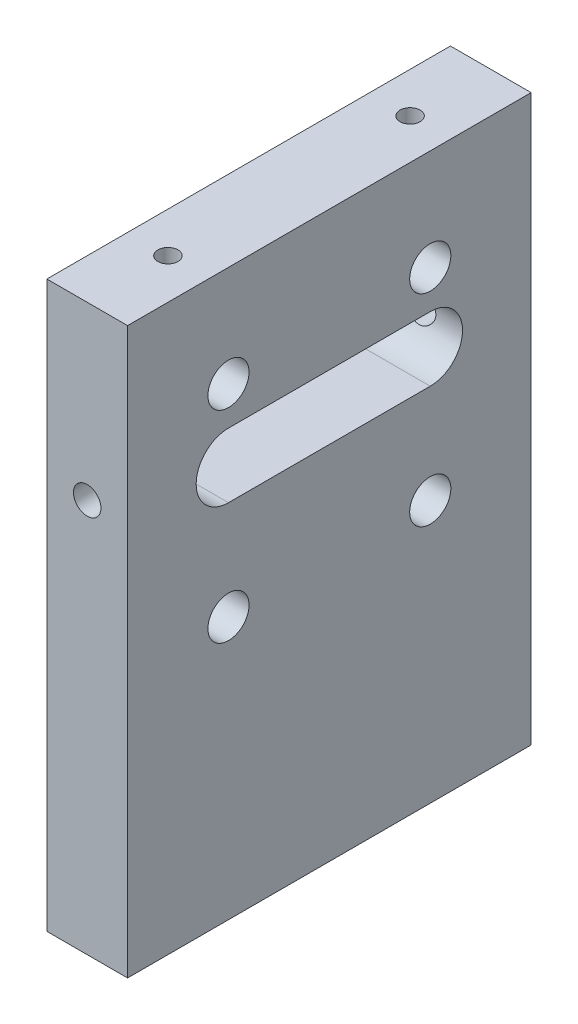
from build123d import *

# Parameters (mm, degrees)
SKETCH_1_W                    = 100
SKETCH_1_H                    = 140
EXTRUDE_1_DEPTH               = 20
HOLE_WIZARD_M6_1_D            = 5
HOLE_WIZARD_M6_1_DEPTH        = 15
HOLE_WIZARD_M6_1_TIP          = 1.502151548
CUT_EXTRUDE_1_DEPTH           = 89.317608663
HOLE_WIZARD_M8_1_D            = 6.8
HOLE_WIZARD_M12_1_D           = 10.2
HOLE_WIZARD_M12_1_CSINK_D     = 12.05
HOLE_WIZARD_M12_1_CSINK_ANGLE = 90
HOLE_WIZARD_M6_2_D            = 5
HOLE_WIZARD_M6_2_DEPTH        = 15
HOLE_WIZARD_M6_2_TIP          = 1.502151548


with BuildPart() as part:
    # 草图1 → 凸台-拉伸1 (new body)
    with BuildSketch(Plane(origin=(0, 0, 0), x_dir=(0, 0, -1), z_dir=(1, 0, 0))):
        Rectangle(SKETCH_1_W, SKETCH_1_H)
    extrude(amount=EXTRUDE_1_DEPTH)

    # M6 螺纹孔1
    with Locations(Plane(origin=(0, -70, 0), x_dir=(-1, 0, 0), z_dir=(0, -1, 0))):
        with Locations((-10, 30), (-10, -30)):
            Hole(HOLE_WIZARD_M6_1_D / 2, depth=HOLE_WIZARD_M6_1_DEPTH)
            with Locations((0, 0, -(HOLE_WIZARD_M6_1_DEPTH + HOLE_WIZARD_M6_1_TIP / 2))):  # 118° drill point
                Cone(0, HOLE_WIZARD_M6_1_D / 2, HOLE_WIZARD_M6_1_TIP, mode=Mode.SUBTRACT)

    # 草图4 → 切除-拉伸1 (cut, through all)
    with BuildSketch(Plane.ZY):
        with BuildLine():
            Line((-25, 35.5), (25, 35.5))
            ThreePointArc((25, 35.5), (33, 27.5), (25, 19.5))
            Line((25, 19.5), (-25, 19.5))
            ThreePointArc((-25, 19.5), (-33, 27.5), (-25, 35.5))
        make_face()
    extrude(amount=-CUT_EXTRUDE_1_DEPTH, mode=Mode.SUBTRACT)

    # M8 螺纹孔1 (through all)
    with Locations(Plane.XY.offset(50)):
        with Locations((10, 27.5)):
            Hole(HOLE_WIZARD_M8_1_D / 2)

    # M12 螺纹孔1 (through all)
    with Locations(Plane.ZY):
        with Locations((-25, 45), (25, 45), (-25, -5), (25, -5)):
            CounterSinkHole(HOLE_WIZARD_M12_1_D / 2, HOLE_WIZARD_M12_1_CSINK_D / 2, counter_sink_angle=HOLE_WIZARD_M12_1_CSINK_ANGLE)

    # M6 螺纹孔2
    with Locations(Plane(origin=(0, 70, 0), x_dir=(1, 0, 0), z_dir=(0, 1, 0))):
        with Locations((10, 30), (10, -30)):
            Hole(HOLE_WIZARD_M6_2_D / 2, depth=HOLE_WIZARD_M6_2_DEPTH)
            with Locations((0, 0, -(HOLE_WIZARD_M6_2_DEPTH + HOLE_WIZARD_M6_2_TIP / 2))):  # 118° drill point
                Cone(0, HOLE_WIZARD_M6_2_D / 2, HOLE_WIZARD_M6_2_TIP, mode=Mode.SUBTRACT)


solid = part.part
